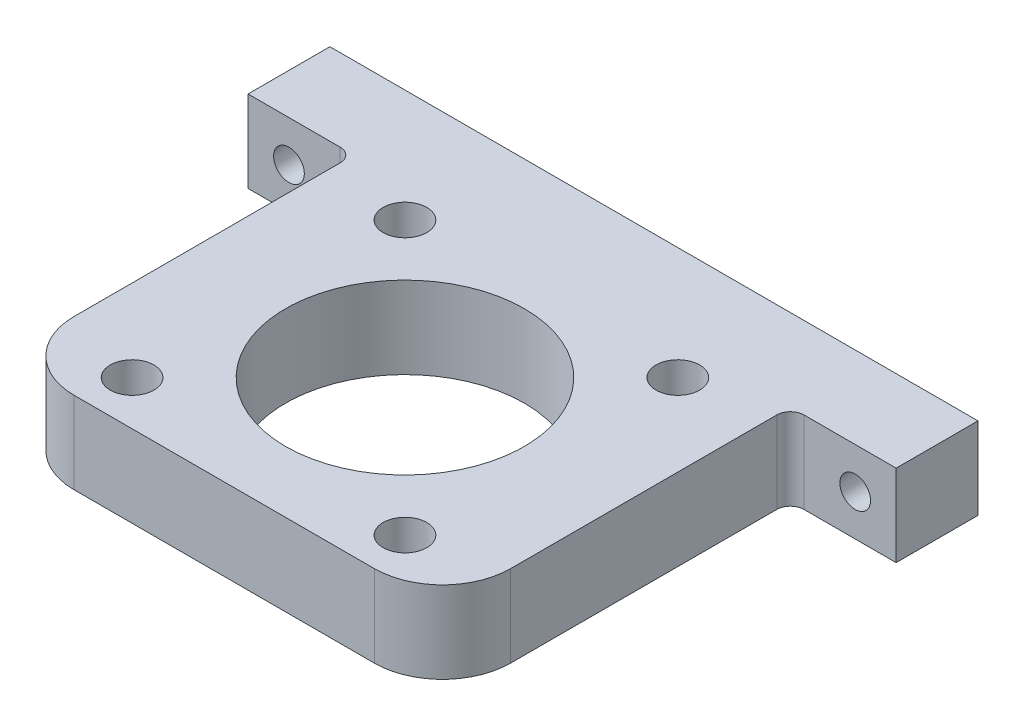
from build123d import *

# Parameters (mm, degrees)
SKETCH_1_W                = 95
SKETCH_1_H                = 63
EXTRUDE_1_DEPTH           = 12
SKETCH_9_W                = 15.5
SKETCH_9_H                = 51
CUT_EXTRUDE_4_DEPTH       = 115.621114983
HOLE_WIZARD_6_5_6_5_1_D   = 4.5
SKETCH_12_R               = 17.5
CUT_EXTRUDE_5_DEPTH       = 115.621114983
FILLET_1_R                = 10
HOLE_WIZARD_5_0_5_1_D     = 5
HOLE_WIZARD_5_0_5_1_DEPTH = 10
HOLE_WIZARD_5_0_5_1_TIP   = 1.502151548
FILLET_2_R                = 2
HOLE_WIZARD_1_D           = 6.4
HOLE_WIZARD_1_CBORE_D     = 11
HOLE_WIZARD_1_CBORE_DEPTH = 7


with BuildPart() as part:
    # 草图1 → 凸台-拉伸1 (new body)
    with BuildSketch(Plane(origin=(0, 0, 0), x_dir=(1, 0, 0), z_dir=(0, 1, 0))):
        with Locations((47.5, -31.5)):
            Rectangle(SKETCH_1_W, SKETCH_1_H)
    extrude(amount=EXTRUDE_1_DEPTH)

    # 草图9 → 切除-拉伸4 (cut, through all)
    with BuildSketch(Plane(origin=(0, 12, 0), x_dir=(1, 0, 0), z_dir=(0, 1, 0))):
        with Locations((7.75, -37.5)):
            Rectangle(SKETCH_9_W, SKETCH_9_H)
        with Locations((87.25, -37.5)):
            Rectangle(SKETCH_9_W, SKETCH_9_H)
    extrude(amount=-CUT_EXTRUDE_4_DEPTH, mode=Mode.SUBTRACT)

    # Ø6.5 (6.5) 直径孔1 (through all)
    with Locations(Plane.XY.offset(12)):
        with Locations((6, 6), (89, 6)):
            Hole(HOLE_WIZARD_6_5_6_5_1_D / 2)

    # 草图12 → 切除-拉伸5 (cut, through all)
    with BuildSketch(Plane(origin=(0, 12, 0), x_dir=(1, 0, 0), z_dir=(0, 1, 0))):
        with Locations(Location((47.5, -36.5, 0), (0, 0, 270))):
            Circle(SKETCH_12_R)
    extrude(amount=-CUT_EXTRUDE_5_DEPTH, mode=Mode.SUBTRACT)

    # 圆角1
    fillet_1_edges = [part.edges().sort_by_distance(p)[0] for p in [
        (15.5, 6, 63),
        (79.5, 6, 63),
    ]]
    fillet(fillet_1_edges, radius=FILLET_1_R)

    # Ø5.0 (5) 直径孔1
    with Locations(Plane(origin=(0, 0, 0), x_dir=(-1, 0, 0), z_dir=(0, 0, -1))):
        with Locations((-67.5, 6), (-27.5, 6)):
            Hole(HOLE_WIZARD_5_0_5_1_D / 2, depth=HOLE_WIZARD_5_0_5_1_DEPTH)
            with Locations((0, 0, -(HOLE_WIZARD_5_0_5_1_DEPTH + HOLE_WIZARD_5_0_5_1_TIP / 2))):  # 118° drill point
                Cone(0, HOLE_WIZARD_5_0_5_1_D / 2, HOLE_WIZARD_5_0_5_1_TIP, mode=Mode.SUBTRACT)

    # 圆角2
    fillet_2_edges = [part.edges().sort_by_distance(p)[0] for p in [
        (15.5, 6, 12),
        (79.5, 6, 12),
    ]]
    fillet(fillet_2_edges, radius=FILLET_2_R)

    # 打孔尺寸(%根据)内六角圆柱头螺钉的类型1 (through all)
    with Locations(Plane(origin=(0, 0, 0), x_dir=(-1, 0, 0), z_dir=(0, -1, 0))):
        with Locations((-67.5, -56.5), (-27.5, -56.5), (-27.5, -16.5), (-67.5, -16.5)):
            CounterBoreHole(HOLE_WIZARD_1_D / 2, HOLE_WIZARD_1_CBORE_D / 2, HOLE_WIZARD_1_CBORE_DEPTH)


solid = part.part
